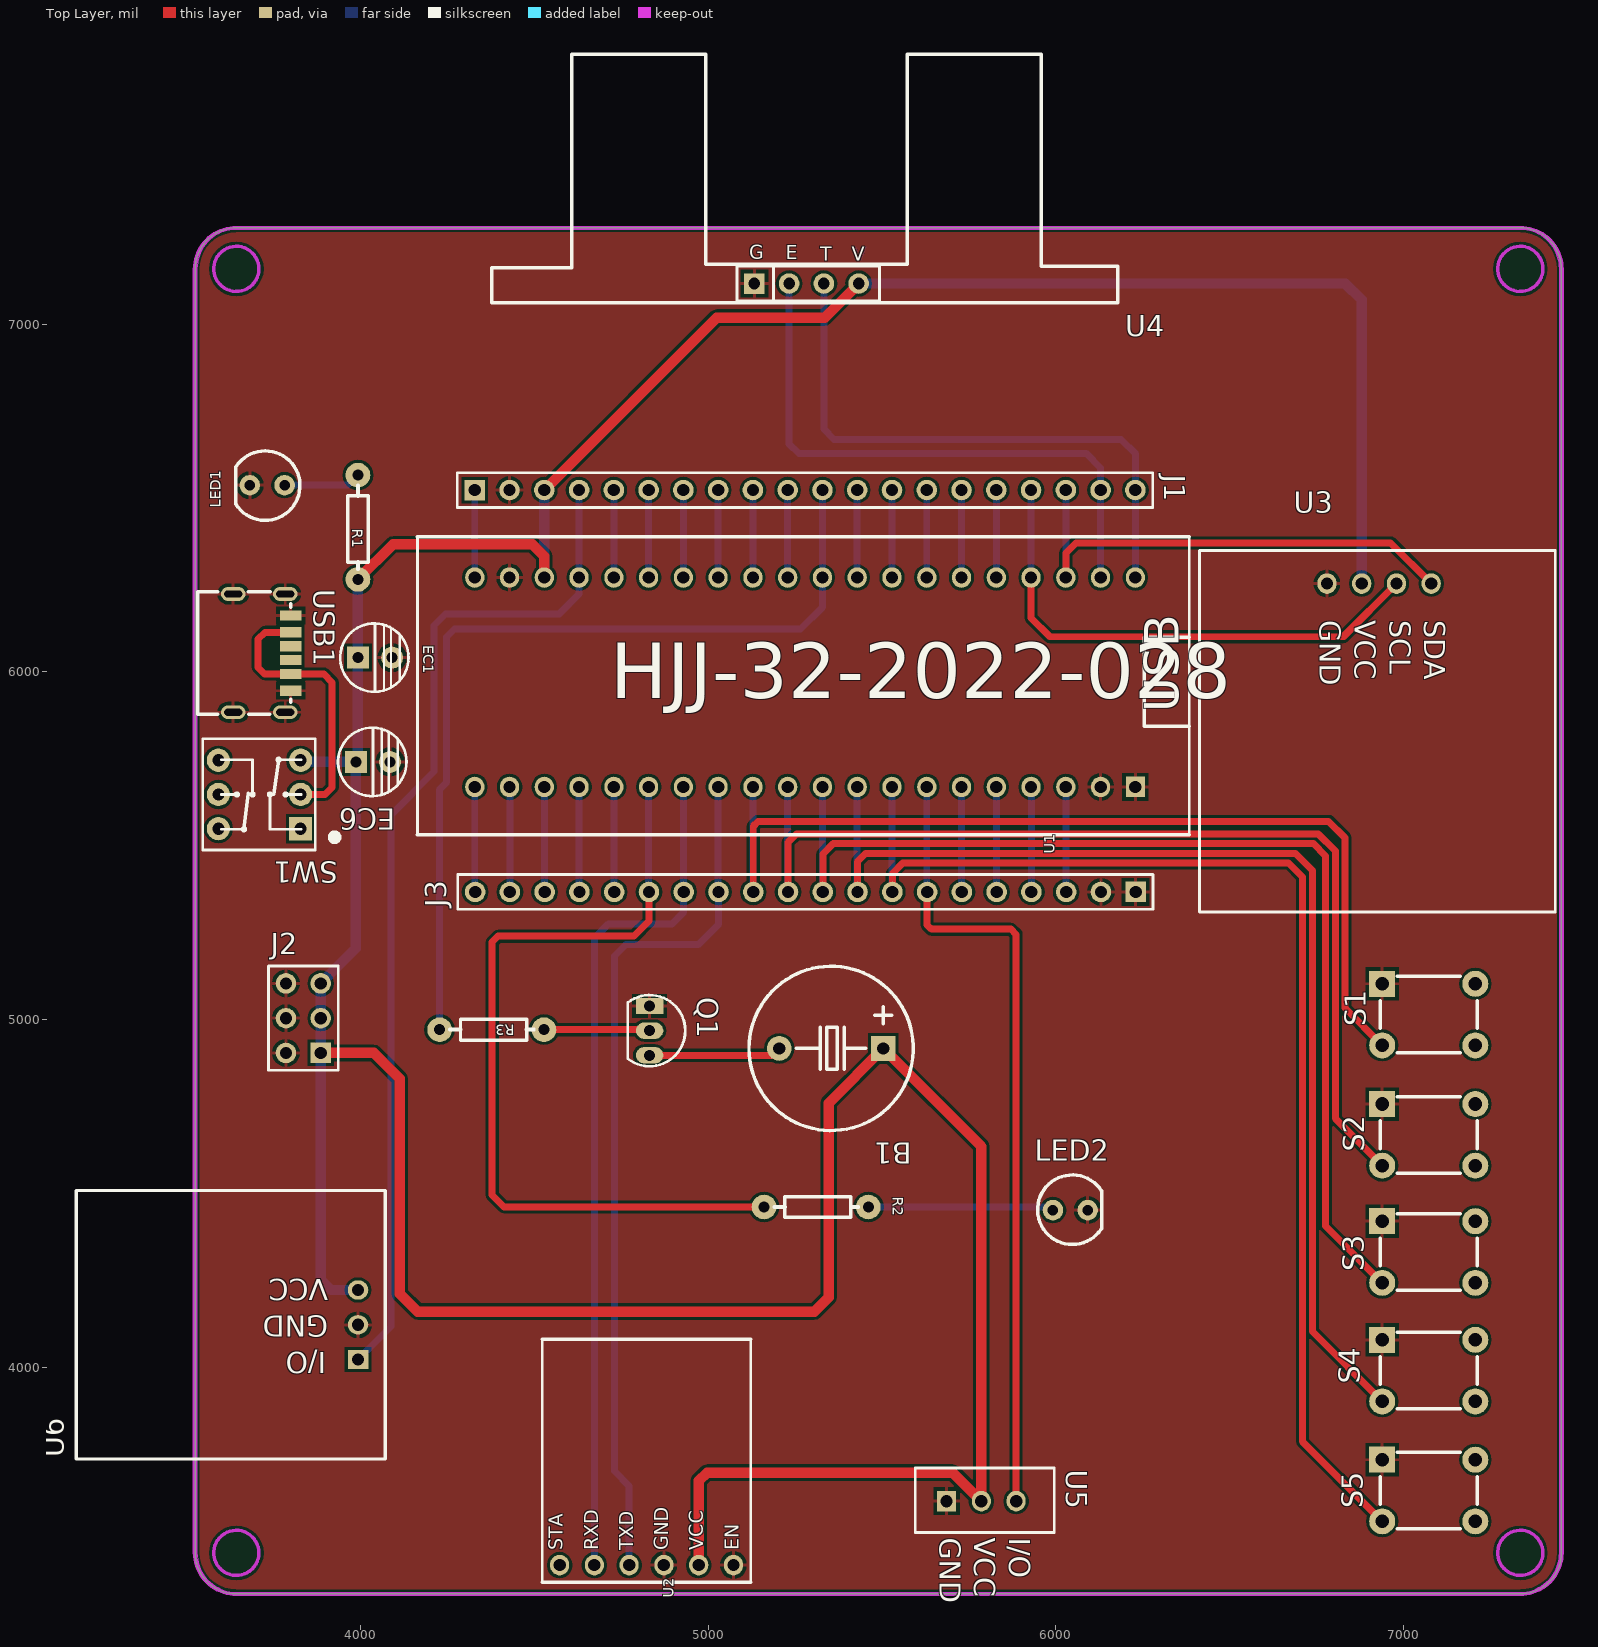
[diagram p0: Top Layer view]
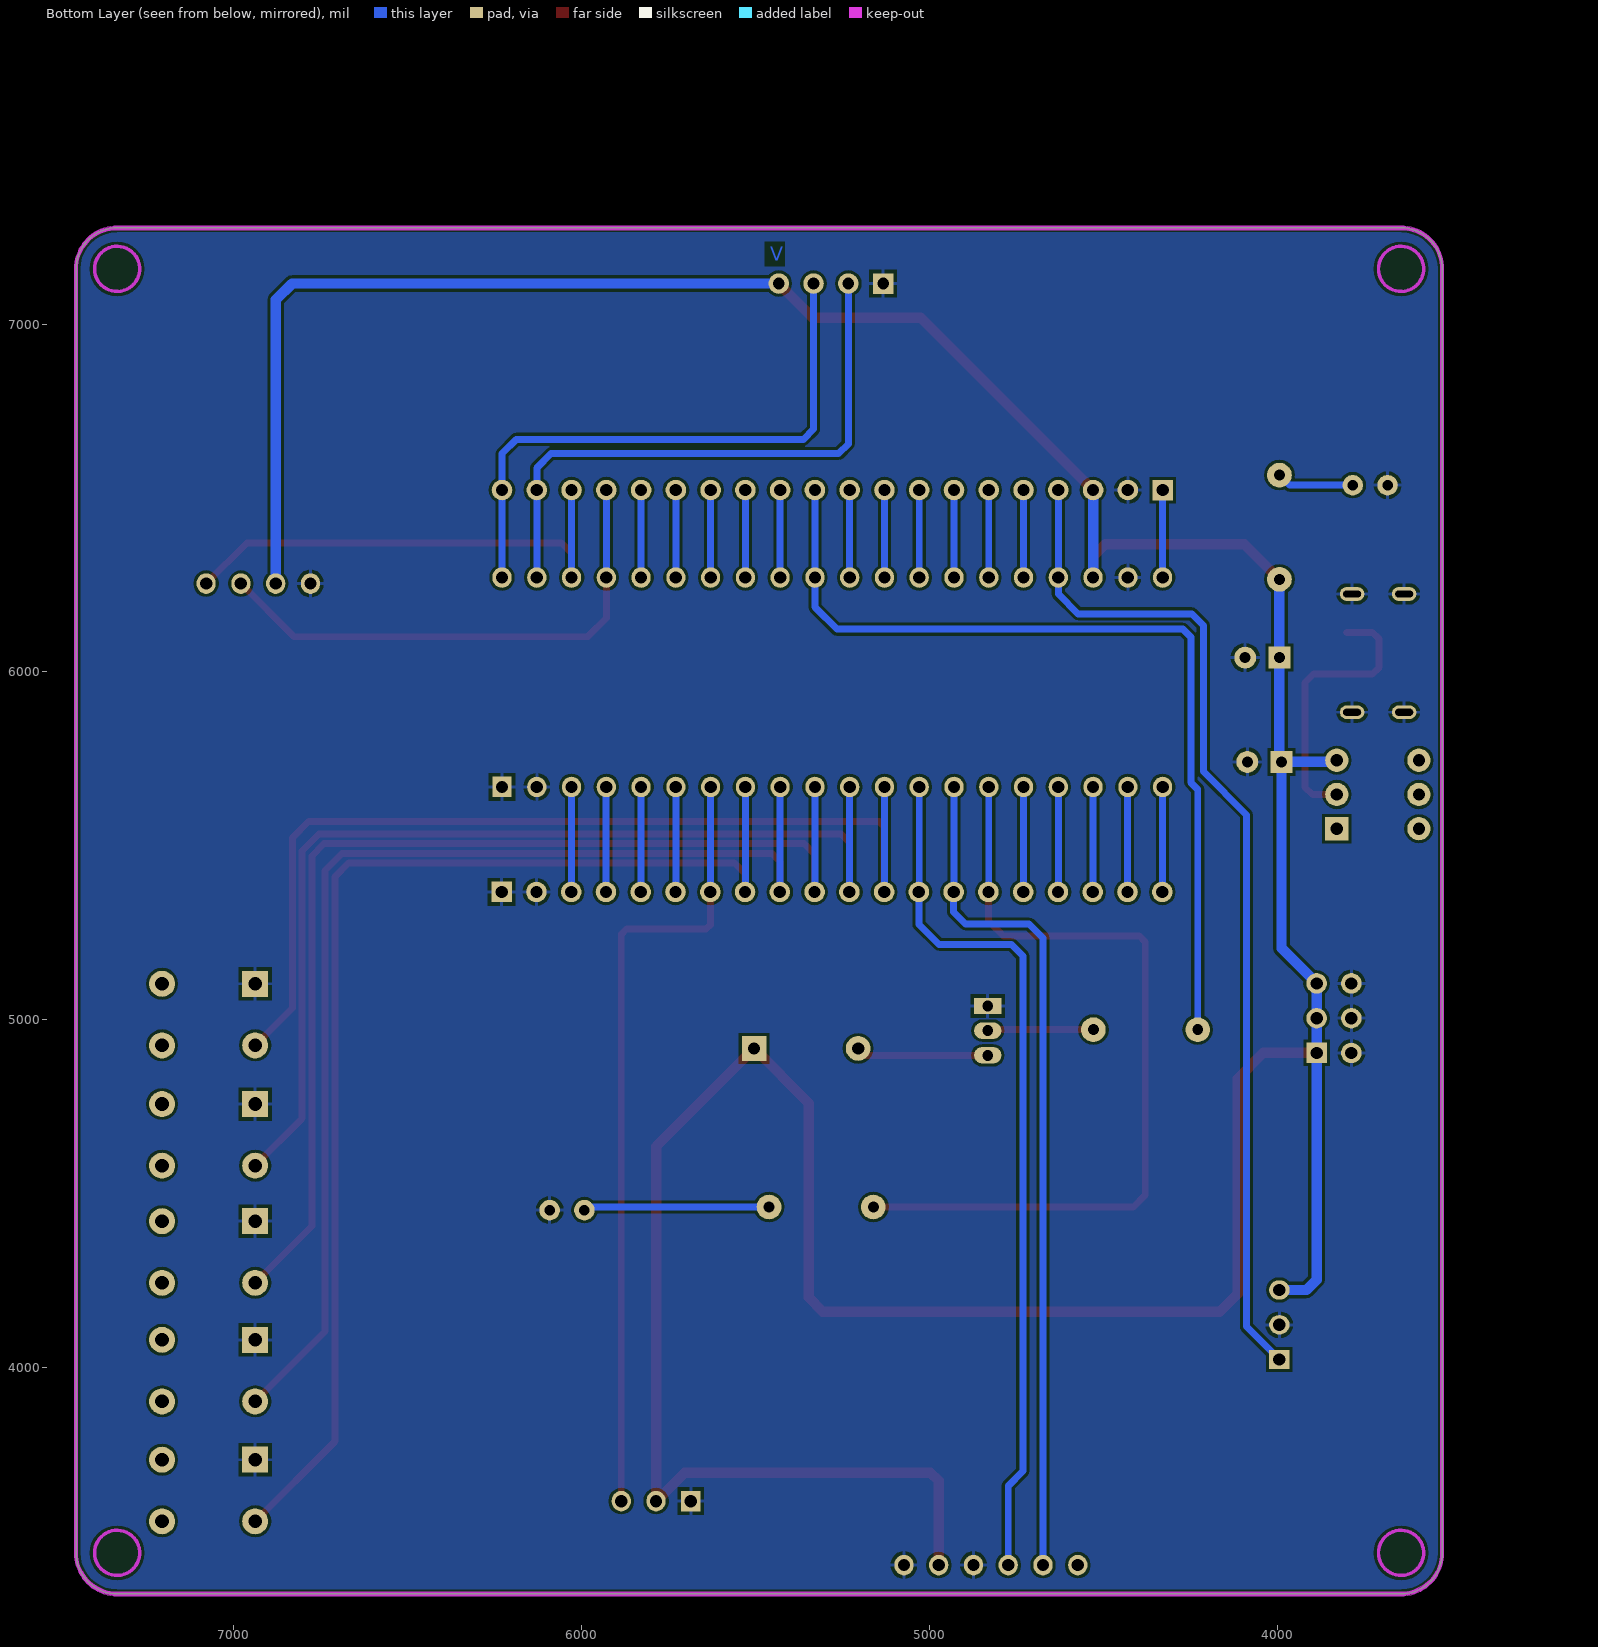
[diagram p1: Bottom Layer view, seen from below]
# Altium PCB MISC51211.pcbdoc
Units mil, origin at the board's own origin, x right, y up, seen from the top; angles counter-clockwise.
Board outline 3929.13 x 3929.13 mil, 2 copper layers (Top Layer, Bottom Layer); 25 components, 43 nets, 161 pads, 0 vias.

## Layer stack, top to bottom (the 12.6 mil dielectric is the usual default, probably not edited)
Top Solder Mask Layer: solder mask 1.4, FR-4, Dk 4.8
Top Layer: signal copper 1.4
Substrate1: surface 12.6, FR-4, Dk 4.8
Bottom Layer: signal copper 1.4
Bottom Solder Mask Layer: solder mask 1.4, FR-4, Dk 4.8

## Board outline
3643.11,3348 cw(c3643.11,3466.11) 3525,3466.11 3525,7159.02 cw(c3643.11,7159.02) 3643.11,7277.13 7336.02,7277.13 cw(c7336.02,7159.02) 7454.13,7159.02 7454.13,3466.11 cw(c7336.02,3466.11) 7336.02,3348

## Design rules (kind name [scope] priority, off if disabled: settings)
BoardOutlineClearance Clearance_1 [All] p2: genericclearance=8 ignorepadtopadclearanceinfootprint=FALSE except(0: Arc-SplitContinuation Track-SplitContinuation SMDPad-SplitContinuation THPad-SplitContinuation Via-SplitContinuation Fill-SplitContinuation Region-SplitContinuation Poly-SplitContinuation Text-SplitContinuation Hole-SplitContinuation; 6: SMDPad-CutoutEdge THPad-CutoutEdge Via-CutoutEdge Fill-CutoutEdge Region-CutoutEdge Text-CutoutEdge; 6.9: Hole-CutoutEdge; 8: Arc-OutlineEdge Track-OutlineEdge SMDPad-OutlineEdge THPad-OutlineEdge Via-OutlineEdge Fill-OutlineEdge Region-OutlineEdge Poly-OutlineEdge Text-OutlineEdge Hole-OutlineEdge Poly-CutoutEdge; 11.8: Arc-CutoutEdge Track-CutoutEdge)
Clearance [All] p1: gap=8 ignorepadtopadclearanceinfootprint=FALSE
DiffPairsRouting [All] p1: maxlimit=10 minlimit=6 mostfreqgap=6 toplayer_minwidth=0 toplayer_prefwidth=0 toplayer_maxwidth=0 toplayer_mingap=10 toplayer_prefgap=10 toplayer_maxgap=10 bottomlayer_minwidth=0 bottomlayer_prefwidth=0 bottomlayer_maxwidth=0 bottomlayer_mingap=10 bottomlayer_prefgap=10 bottomlayer_maxgap=10 maxuncoupledlength=10
HoleToHoleClearance ComponentClearance [All] p1: gap=10 allowstackedmicrovias=TRUE
Length netLength [All] p1: minlimit=0 maxlimit=0
MatchedLengths netLengthTolerance [All] p1: tolerance=1000
PolygonConnect [All] p1: connectstyle=Relief reliefconductorwidth=10 reliefentries=4 polygonreliefangle="90 Angle" airgapwidth=10 via.connectstyle=Relief via.reliefconductorwidth=10 via.reliefentries=4 via.polygonreliefangle="90 Angle" via.airgapwidth=10
RoutingVias [All] p1: holewidth=11.81 width=23.62 viastyle="Through Hole" minholewidth=11.81 minwidth=23.62 maxholewidth=11.81 maxwidth=23.62
SolderMaskExpansion [All] p1: expansion=4 istentingtop=FALSE
Width [All] p1: maxlimit=10 minlimit=10 preferedwidth=10 toplayer_minwidth=20 toplayer_maxwidth=30 toplayer_prefwidth=20 bottomlayer_minwidth=20 bottomlayer_maxwidth=30 bottomlayer_prefwidth=20
2 further rules are at their usual default settings.

## Components (designator, comment, footprint, x,y, rotation, side; value= is the part's Value field where it differs from the comment)
B1 "BEEP" "BEEP 7.6X12X7.5" 5504,4917 r180 top
EC1 "220uF" DIP-EC2.5X5X11 3993,6041 r0 top
EC6 "10uF" DIP-EC2.5X5X11 3987,5741 r0 top
J1 "" "Pin HDR1X20/2.54mm-S" 4329,6523 r0 top
J2 "Pin HDR2X3" "Pin HDR2X3/2.54mm-S" 3886,4904 r90 top
J3 "" "Pin HDR1X20/2.54mm-S" 6230,5367 r180 top
LED1 "LED" LED5-BLUE 3732,6537 r180 top
LED2 "LED" LED5-BLUE 6042,4452 r0 top
Q1 "NPN" TO-92A 4832,5039 r270 top
R1 "1k" AXIAL0.3 3993,6566 r270 top
R2 "k?" AXIAL0.3 5161,4461 r0 top
R3 "1K" AXIAL0.3 4228,4971 r0 top
S1 "BUTTOM" DIP-6X6X5 6939,5103 r0 top
S2 "BUTTOM" DIP-6X6X5 6939,4757 r0 top
S3 "BUTTOM" DIP-6X6X5 6939,4420 r0 top
S4 "BUTTOM" DIP-6X6X5 6939,4079 r0 top
S5 "BUTTOM" DIP-6X6X5 6939,3734 r0 top
SW1 "KFT DIP-8X8" "KFT DIP-8X8" 3828,5549 r180 top
U1 "STM32F103" STM32FF103 6229,5669 r90 top
U2 "ESP8266" ECB02 5123,3381 r90 top
U3 "OLED" OLED 6925,6254 r270 top
U4 "HC-SR04" 超声波MODE 5283,7062 r0 top
U5 "SG90" SG90 5686,3615 r270 top
U6 "Infrared pair" 红外对管 4072,4508 r180 top
USB1 "TYPEC-250D-BCP6" TYP-C-6 3717,6054 r270 top

## Footprints (in the part's own frame and the unit in brackets; to place one, negate y for a bottom-side part, rotate by r counter-clockwise, add the part's x,y. Pads: shape width x height; smd on the part's side, far side on the other; paste and mask are expansions set on the pad)
AXIAL0.3 [mm]
  round 1.8 hole 0.8: 1(0,0) 2(7.62,0)
  silkscreen extent 0.76,-0.76 6.86,0.76
"BEEP 7.6X12X7.5" [mm]
  rect 1.8x1.8 hole 0.9: 1(0,0)
  round 1.8 hole 0.9: 2(7.6,0)
  silkscreen extent -2.19,-6 9.81,6
DIP-6X6X5 [mm]
  rect 1.9x1.9 hole 1: 1(0,0)
  round 1.9 hole 1: 2(0,-4.5) 3(6.8,-4.5) 4(6.8,0)
  silkscreen extent -0.16,-5.04 6.96,0.54
DIP-EC2.5X5X11 [mm]
  rect 1.6x1.6 hole 0.8: 1(0,0)
  round 1.6 hole 0.8: 2(2.5,0)
  silkscreen extent -1.3,-2.5 3.7,2.5
ECB02 [mm]
  oval 1.5x1.4 hole 0.9: 1(1.27,13.97) 2(1.27,11.43) 3(1.27,8.89) 4(1.27,6.35) 5(1.27,3.81) 6(1.27,1.27)
  silkscreen extent 0,0 17.78,15.24
"KFT DIP-8X8" [mm]
  rect 1.7x1.7 hole 0.9: 1(0,0)
  round 1.7 hole 0.9: 2(0,-2.5) 3(0,-5) 4(6,-5) 5(6,-2.5) 6(6,0)
  silkscreen extent -2.69,-6.56 7.15,1.56
LED5-BLUE [mm]
  round 1.5 hole 0.762: A(-1.27,0) K(1.27,0)
  silkscreen extent -2.39,-2.51 2.29,2.57
OLED [mm]
  oval 1.5x1.4 hole 0.9: 1(0,-3.683) 2(0,-1.143) 3(0,1.397) 4(0,3.937)
  silkscreen extent -2.41,-13 24,13
"Pin HDR1X20/2.54mm-S" [mm]
  rect 1.5x1.5 hole 0.9: 1(0,0)
  round 1.5 hole 0.9: 2(2.54,0) 3(5.08,0) 4(7.62,0) 5(10.16,0) 6(12.7,0) 7(15.24,0) 8(17.78,0) 9(20.32,0) 10(22.86,0) 11(25.4,0) 12(27.94,0) 13(30.48,0) 14(33.02,0) 15(35.56,0) 16(38.1,0) 17(40.64,0) 18(43.18,0) 19(45.72,0) 20(48.26,0)
  silkscreen extent -1.27,-1.27 49.53,1.27
"Pin HDR2X3/2.54mm-S" [mm]
  rect 1.5x1.5 hole 0.9: 1(0,0)
  round 1.5 hole 0.9: 2(0,2.54) 3(2.54,0) 4(2.54,2.54) 5(5.08,0) 6(5.08,2.54)
  silkscreen extent -1.27,-1.27 6.35,3.81
SG90 [mm]
  rect 1.5x1.4 hole 0.9: 1(0,0)
  oval 1.5x1.4 hole 0.9: 2(0,2.54) 3(0,5.08)
  silkscreen extent -2.41,-2.29 2.29,7.87
STM32FF103 [mm]
  rect 1.5x1.4 hole 0.9: 1(0,0)
  oval 1.5x1.4 hole 0.9: 2(0,2.54) 3(0,5.08) 4(0,7.62) 5(0,10.16) 6(0,12.7) 7(0,15.24) 8(0,17.78) 9(0,20.32) 10(0,22.86) 11(0,25.4) 12(0,27.94) 13(0,30.48) 14(0,33.02) 15(0,35.56) 16(0,38.1) 17(0,40.64) 18(0,43.18) 19(0,45.72) 20(0,48.26) 25(15.3,48.26) 26(15.3,45.72) 27(15.3,43.18) 28(15.3,40.64) 29(15.3,38.1) 30(15.3,35.56) 31(15.3,33.02) 32(15.3,30.48) 33(15.3,27.94) 34(15.3,25.4) 35(15.3,22.86) 36(15.3,20.32) 37(15.3,17.78) 38(15.3,15.24) 39(15.3,12.7) 40(15.3,10.16) 41(15.3,7.62) 42(15.3,5.08) 43(15.3,2.54) 44(15.3,0)
  silkscreen extent -3.5,-3.94 18.29,52.45
TO-92A [mm]
  oval 1.2x2 hole 0.8: B(1.8,0) C(3.6,0)
  rect 1.2x2 hole 0.8: E(0,0)
  silkscreen extent -0.8,-1.6 4.4,2.6
TYP-C-6 [mm]
  oval 1x1.8 hole 0.5 slot 1.3 at 90 deg: 1(-4.32,1.7) 2(-4.32,-2.1) 3(4.32,-2.1) 4(4.32,1.7)
  rect 0.75x1.6 smd: A5(-0.5,2.1) A9(1.52,2.1) A12(2.75,2.1) B5(0.5,2.1) B9(-1.52,2.1) B12(-2.75,2.1)
  silkscreen extent -4.48,-4.7 4.47,2.1
红外对管 [mm]
  rect 1.5x1.4 hole 0.9: 1(2,12.34)
  oval 1.5x1.4 hole 0.9: 2(2,9.8) 3(2,7.26)
  silkscreen extent 0,0 22.6,19.6
超声波MODE [mm]
  rect 1.5x1.5 hole 0.85: 1(-3.81,1.397)
  round 1.5 hole 0.85: 2(-1.27,1.397) 3(1.27,1.397) 4(3.81,1.397)
  silkscreen extent -22.99,0 22.73,18.16

## Nets (pads, with @x,y where several pads share a name; then routed paths per layer and width w, separated by ;. In a path a pad name is that pad's centre, name@x,y a point inside that pad or via, vN(x,y) a via of type N, cw(c..) or ccw(c..) an arc to the next point about the centre after c; other vN are vias at no path point)
ECHO: J1.19 U1.43 U4.2 | length 1701.2
  Bottom Layer w20: U4.2 5233,6656 5261,6628 6088,6628 6129,6587 J1.19 U1.43
GND: EC1.2 EC6.2 J1.2 J2.2 J2.4 J2.6 J3.1 J3.2 LED1.K LED2.K Q1.E S1.1 S2.1 S3.1 S4.1 S5.1 U1.1 U1.2 U1.26 U2.4 U2.6 U3.1 U4.1 U5.1 U6.2 USB1.1 USB1.2 USB1.3 USB1.4 USB1.A12 USB1.B12
NetB1_2: B1.2 Q1.C | length 381
  Top Layer w20: Q1.C 5185.06,4897.27 B1.2
NetJ1_1: J1.1 U1.25 | length 251.6
  Bottom Layer w20: U1.25 J1.1
NetLED1_A: LED1.A R1.1 | length 223
  Bottom Layer w20: LED1.A 3964,6537 R1.1
NetLED2_A: LED2.A R2.2 | length 534.7
  Bottom Layer w20: R2.2 5983,4461 LED2.A
NetQ1_B: Q1.B R3.2 | length 305.2
  Top Layer w20: R3.2 4829.13,4971 Q1.B
PA0: J3.16 U1.16 | length 301
  Bottom Layer w20: J3.16@4729,5368 U1.16
PA1: J3.15 R2.1 U1.15 | length 2384.9
  Top Layer w20: J3.15 4830,5283 4787,5240 4396,5240 4379,5223 4379,4495 4413,4461 R2.1
  Bottom Layer w20: J3.15@4829,5368 U1.15
PA2: J3.14 U1.14 U2.2 | length 2450.7
  Bottom Layer w20: U2.2 4673,5235 4713,5275 4896,5275 4930,5309 J3.14 ; J3.14@4929,5368 U1.14
PA3: J3.13 U1.13 U2.3 | length 2500.1
  Bottom Layer w20: U2.3 4773,3659 4731,3701 4731,5183 4764,5216 4972,5216 5030,5274 J3.13 ; J3.13@5029,5368 U1.13
PA4: J3.12 S1.2 U1.12 | length 2858.8
  Top Layer w20: J3.12 5130,5556 5144,5570 6785,5570 6832,5523 6832,5032.83 S1.2
  Bottom Layer w20: J3.12@5129,5368 U1.12
PA5: J3.11 S2.2 U1.11 | length 3009.3
  Top Layer w20: J3.11 5230,5510 5254,5534 6755,5534 6804,5485 6804,4714.83 S2.2
  Bottom Layer w20: J3.11@5229,5368 U1.11
PA6: J3.10 S3.2 U1.10 | length 3178.6
  Top Layer w20: J3.10 5330,5476 5360,5506 6741,5506 6776,5471 6776,4405.83 S3.2
  Bottom Layer w20: J3.10@5329,5368 U1.10
PA7: J3.9 S4.2 U1.9 | length 3337.2
  Top Layer w20: J3.9 5430,5455 5453,5478 6689,5478 6738,5429 6738,4102.83 S4.2
  Bottom Layer w20: J3.9@5429,5368 U1.9
PA8: J1.16 U1.40 | length 251.6
  Bottom Layer w20: U1.40 J1.16
PA9: J1.15 U1.39 | length 251.6
  Bottom Layer w20: U1.39 J1.15
PA10: J1.14 U1.38 | length 251.6
  Bottom Layer w20: U1.38 J1.14
PA11: J1.13 U1.37 | length 251.6
  Bottom Layer w20: U1.37 J1.13
PA12: J1.12 U1.36 | length 251.6
  Bottom Layer w20: U1.36 J1.12
PA15: J1.11 R3.1 U1.35 | length 2590.9
  Bottom Layer w20: R3.1 4228,5662 4248,5682 4248,6100 4271,6123 5266,6123 5329,6186 U1.35 J1.11
PB0: J3.8 S5.2 U1.8 | length 3511
  Top Layer w20: J3.8 5530,5420 5560,5450 6670,5450 6710,5410 6710,3785.83 S5.2
  Bottom Layer w20: J3.8@5529,5368 U1.8
PB1: J3.7 U1.7 U5.3 | length 2293.2
  Top Layer w20: J3.7 5630,5272 5642,5260 5871,5260 5886,5245 U5.3
  Bottom Layer w20: J3.7@5629,5368 U1.7
PB3: J1.10 U1.34 | length 251.6
  Bottom Layer w20: U1.34 J1.10
PB4: J1.9 U1.33 | length 251.6
  Bottom Layer w20: U1.33 J1.9
PB5: J1.8 U1.32 | length 251.6
  Bottom Layer w20: U1.32 J1.8
PB6: J1.7 U1.31 | length 251.6
  Bottom Layer w20: U1.31 J1.7
PB7: J1.6 U1.30 | length 251.6
  Bottom Layer w20: U1.30 J1.6
PB8: J1.5 U1.29 | length 251.6
  Bottom Layer w20: U1.29 J1.5
PB9: J1.4 U1.28 U6.1 | length 2955.7
  Bottom Layer w20: U6.1 4088,4116.91 4088,5589 4212,5713 4212,6134 4245,6167 4572,6167 4629,6224 U1.28 J1.4
PB10: J3.6 U1.6 | length 301
  Bottom Layer w20: J3.6@5729,5368 U1.6
PB11: J3.5 U1.5 | length 301
  Bottom Layer w20: J3.5@5829,5368 U1.5
PB12: J1.20 U1.44 U4.3 | length 1700.6
  Bottom Layer w20: U4.3 5333,6698 5362,6669 6188,6669 6229,6628 J1.20 U1.44
PB14: J1.18 U1.42 U3.4 | length 1433.8
  Top Layer w20: U1.42 6029,6342 6058,6371 6963,6371 U3.4
  Bottom Layer w20: U1.42 J1.18
PB15: J1.17 U1.41 U3.3 | length 1504.7
  Top Layer w20: U1.41 5929,6155 5983,6101 6827,6101 U3.3
  Bottom Layer w20: U1.41 J1.17
PC13: J3.19 U1.19 | length 301
  Bottom Layer w20: J3.19 U1.19@4430,5668
PC14: J3.18 U1.18 | length 301
  Bottom Layer w20: J3.18@4529,5368 U1.18
PC15: J3.17 U1.17 | length 301
  Bottom Layer w20: J3.17@4629,5368 U1.17
R: J3.4 U1.4 | length 301
  Bottom Layer w20: J3.4 U1.4@5930,5668
VB: J3.20 U1.20 | length 301
  Bottom Layer w20: J3.20@4329,5368 U1.20
VCC: B1.1 EC1.1 EC6.1 J1.3 J2.1 J2.3 J2.5 R1.2 SW1.3 U1.27 U2.5 U3.2 U4.4 U5.2 U6.3 | length 12123
  Top Layer w30: J2.1 4039,4904 4113,4830 4113,4212 4165,4160 5306,4160 5347,4201 5347,4760 B1.1 5786,4635 U5.2 5704,3697 4997,3697 4973,3673 U2.5 ; R1.2 4094,6367 4494,6367 4529,6332 U1.27 ; J1.3 5025,7019 5335,7019 U4.4
  Bottom Layer w30: SW1.3 3832.85,5741 EC6.1 ; R1.2 EC1.1 3993,5747 EC6.1 ; U6.3 3915.83,4222.17 3886,4252 J2.1 J2.3 J2.5 3987,5205 EC6.1 ; U1.27 J1.3 ; U4.4 6833,7117 6880,7070 U3.2
VCC_3V3: J3.3 U1.3 | length 301
  Bottom Layer w20: J3.3@6029,5368 U1.3
VIN: SW1.2 USB1.A9 USB1.B9 | length 815.2
  Top Layer w20: USB1.B9 3725.85,6113.85 3706,6094 3706,6013 3724.84,5994.16 USB1.A9 3894.84,5994.16 3919,5970 3919,5668 3898.43,5647.43 SW1.2
pads on no net: S1.3 S1.4 S2.3 S2.4 S3.3 S3.4 S4.3 S4.4 S5.3 S5.4 SW1.1 SW1.4 SW1.5 SW1.6 U2.1 USB1.A5 USB1.B5

## Polygon pours and split planes (outlines as drawn)
GND on Top Layer (solid, remove dead copper, pour order 8): 3208,7378 3260,7430 7664,7430 7664,3061 7612,3009 7516,3105 3000,3105
GND on Bottom Layer (solid, remove dead copper, pour order 14): 3078,7439 3104,7413 7847,7413 7847,3070 7777,3000 7690,3087 3061,3087

## Keep-outs
Board Outline Layer:
  region: 3708.07,7159.02 cw(c3643.11,7159.02) 3578.15,7159.02 cw(c3643.11,7159.02)
  circle w10: c3643.11,7159.02 r64.96
  region: 7400.98,7159.02 cw(c7336.02,7159.02) 7271.06,7159.02 cw(c7336.02,7159.02)
  circle w10: c7336.02,7159.02 r64.96
  region: 7400.98,3466.11 cw(c7336.02,3466.11) 7271.06,3466.11 cw(c7336.02,3466.11)
  circle w10: c7336.02,3466.11 r64.96
  region: 3708.07,3466.11 cw(c3643.11,3466.11) 3578.15,3466.11 cw(c3643.11,3466.11)
  circle w10: c3643.11,3466.11 r64.96
  region: 3643.11,3343 3633.45,3343.38 3623.85,3344.52 3614.37,3346.4 3605.07,3349.03 3596,3352.37 3587.22,3356.42 3578.79,3361.14 3570.75,3366.51 3563.16,3372.5 3556.06,3379.06 3549.5,3386.16 3543.51,3393.75 3538.14,3401.79 3533.42,3410.22 3529.37,3419 3526.03,3428.07 3523.4,3437.37 3521.52,3446.85 3520.38,3456.45 3520,3466.11 3520.38,3468.02 3521.46,3469.65 3523.09,3470.73 3525,3471.11 3526.91,3470.73 3528.54,3469.65 3529.62,3468.02 3530,3466.11 3530.39,3456.77 3531.54,3447.49 3533.46,3438.34 3536.13,3429.38 3539.53,3420.67 3543.63,3412.28 3548.42,3404.24 3553.85,3396.64 3559.89,3389.5 3566.5,3382.89 3573.64,3376.85 3581.24,3371.42 3589.28,3366.63 3597.67,3362.53 3606.38,3359.13 3615.34,3356.46 3624.49,3354.54 3633.77,3353.39 3643.11,3353 3645.02,3352.62 3646.65,3351.54 3647.73,3349.91 3648.11,3348 3647.73,3346.09 3646.65,3344.46 3645.02,3343.38
  region: 3530,7159.02 3529.62,7157.11 3528.54,7155.49 3526.91,7154.4 3525,7154.02 3523.09,7154.4 3521.46,7155.49 3520.38,7157.11 3520,7159.02 3520.38,7168.68 3521.52,7178.28 3523.4,7187.76 3526.03,7197.07 3529.37,7206.14 3533.42,7214.91 3538.14,7223.35 3543.51,7231.39 3549.5,7238.98 3556.06,7246.08 3563.16,7252.64 3570.75,7258.62 3578.79,7263.99 3587.22,7268.72 3596,7272.76 3605.07,7276.11 3614.37,7278.73 3623.85,7280.62 3633.45,7281.75 3643.11,7282.13 3645.02,7281.75 3646.65,7280.67 3647.73,7279.05 3648.11,7277.13 3647.73,7275.22 3646.65,7273.6 3645.02,7272.51 3643.11,7272.13 3633.77,7271.75 3624.49,7270.59 3615.34,7268.67 3606.38,7266.01 3597.67,7262.61 3589.28,7258.5 3581.24,7253.72 3573.64,7248.28 3566.5,7242.24 3559.89,7235.63 3553.85,7228.5 3548.42,7220.89 3543.63,7212.86 3539.53,7204.46 3536.13,7195.75 3533.46,7186.79 3531.54,7177.64 3530.39,7168.36
  region: 7459.13,7159.02 7458.75,7157.11 7457.67,7155.49 7456.05,7154.4 7454.13,7154.02 7452.22,7154.4 7450.6,7155.49 7449.51,7157.11 7449.13,7159.02 7448.75,7168.36 7447.59,7177.64 7445.67,7186.79 7443.01,7195.75 7439.61,7204.46 7435.5,7212.86 7430.72,7220.89 7425.28,7228.5 7419.24,7235.63 7412.63,7242.24 7405.5,7248.28 7397.89,7253.72 7389.86,7258.5 7381.46,7262.61 7372.75,7266.01 7363.79,7268.67 7354.64,7270.59 7345.36,7271.75 7336.02,7272.13 7334.11,7272.51 7332.49,7273.6 7331.4,7275.22 7331.02,7277.13 7331.4,7279.05 7332.49,7280.67 7334.11,7281.75 7336.02,7282.13 7345.68,7281.75 7355.28,7280.62 7364.76,7278.73 7374.07,7276.11 7383.14,7272.76 7391.91,7268.72 7400.35,7263.99 7408.39,7258.62 7415.98,7252.64 7423.08,7246.08 7429.64,7238.98 7435.62,7231.39 7440.99,7223.35 7445.72,7214.91 7449.76,7206.14 7453.11,7197.07 7455.73,7187.76 7457.62,7178.28 7458.75,7168.68 7459.13,7159.02
  region: 7459.13,3466.11 7458.75,3456.45 7457.62,3446.85 7455.73,3437.37 7453.11,3428.07 7449.76,3419 7445.72,3410.22 7440.99,3401.79 7435.62,3393.75 7429.64,3386.16 7423.08,3379.06 7415.98,3372.5 7408.39,3366.51 7400.35,3361.14 7391.91,3356.42 7383.14,3352.37 7374.07,3349.03 7364.76,3346.4 7355.28,3344.52 7345.68,3343.38 7336.02,3343 7334.11,3343.38 7332.49,3344.46 7331.4,3346.09 7331.02,3348 7331.4,3349.91 7332.49,3351.54 7334.11,3352.62 7336.02,3353 7345.36,3353.39 7354.64,3354.54 7363.79,3356.46 7372.75,3359.13 7381.46,3362.53 7389.86,3366.63 7397.89,3371.42 7405.5,3376.85 7412.63,3382.89 7419.24,3389.5 7425.28,3396.64 7430.72,3404.24 7435.5,3412.28 7439.61,3420.67 7443.01,3429.38 7445.67,3438.34 7447.59,3447.49 7448.75,3456.77 7449.13,3466.11 7449.51,3468.02 7450.6,3469.65 7452.22,3470.73 7454.13,3471.11 7456.05,3470.73 7457.67,3469.65 7458.75,3468.02 7459.13,3466.11
  region: 7454.13,3461.11 7452.22,3461.49 7450.6,3462.57 7449.51,3464.2 7449.13,3466.11 7449.13,7159.02 7449.51,7160.94 7450.6,7162.56 7452.22,7163.64 7454.13,7164.02 7456.05,7163.64 7457.67,7162.56 7458.75,7160.94 7459.13,7159.02 7459.13,3466.11 7458.75,3464.2 7457.67,3462.57 7456.05,3461.49
  region: 3525,3461.11 3523.09,3461.49 3521.46,3462.57 3520.38,3464.2 3520,3466.11 3520,7159.02 3520.38,7160.94 3521.46,7162.56 3523.09,7163.64 3525,7164.02 3526.91,7163.64 3528.54,7162.56 3529.62,7160.94 3530,7159.02 3530,3466.11 3529.62,3464.2 3528.54,3462.57 3526.91,3461.49
  region: 7341.02,7277.13 7340.64,7275.22 7339.56,7273.6 7337.94,7272.51 7336.02,7272.13 3643.11,7272.13 3641.2,7272.51 3639.57,7273.6 3638.49,7275.22 3638.11,7277.13 3638.49,7279.05 3639.57,7280.67 3641.2,7281.75 3643.11,7282.13 7336.02,7282.13 7337.94,7281.75 7339.56,7280.67 7340.64,7279.05
  region: 7341.02,3348 7340.64,3346.09 7339.56,3344.46 7337.94,3343.38 7336.02,3343 3643.11,3343 3641.2,3343.38 3639.57,3344.46 3638.49,3346.09 3638.11,3348 3638.49,3349.91 3639.57,3351.54 3641.2,3352.62 3643.11,3353 7336.02,3353 7337.94,3352.62 7339.56,3351.54 7340.64,3349.91
  lines w10: 3525,3466.11 ccw(c3643.11,3466.11) 3643.11,3348 7336.02,3348 ccw(c7336.02,3466.11) 7454.13,3466.11 7454.13,7159.02 ccw(c7336.02,7159.02) 7336.02,7277.13 3643.11,7277.13 ccw(c3643.11,7159.02) 3525,7159.02 3525,3466.11